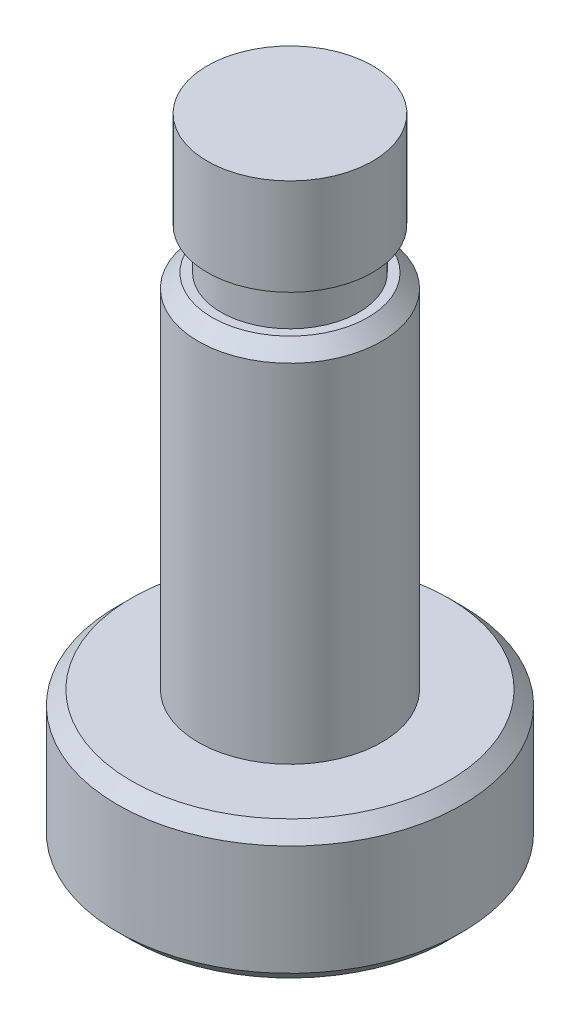
from build123d import *

# Parameters (mm, degrees)
CHAMFER_1_SIZE = 1


with BuildPart() as part:
    # 草图1 → 旋转1 (revolve)
    with BuildSketch(Plane.XY, mode=Mode.PRIVATE) as revolve_1_sk:
        Polygon((349.087142185, 76.281973739), (349.087142185, 69.281973739), (348.087142185, 69.281973739), (348.087142185, 66.281973739), (349.737142185, 66.281973739), (349.737142185, 40.081973739), (355.587142185, 40.081973739), (355.587142185, 30.081973739), (343.087142185, 30.081973739), (343.087142185, 76.281973739), align=None)
    revolve(revolve_1_sk.sketch.rotate(Axis((343.087142185, 30.081973739, 0), (0, 1, 0)), 90), axis=Axis((343.087142185, 30.081973739, 0), (0, 1, 0)))

    # 倒角1
    chamfer_1_edges = [part.edges().sort_by_distance(p)[0] for p in [
        (343.087142185, 66.281973739, 6.65),
        (343.087142185, 30.081973739, 12.5),
        (343.087142185, 40.081973739, 12.5),
    ]]
    chamfer(chamfer_1_edges, length=CHAMFER_1_SIZE)


solid = part.part
